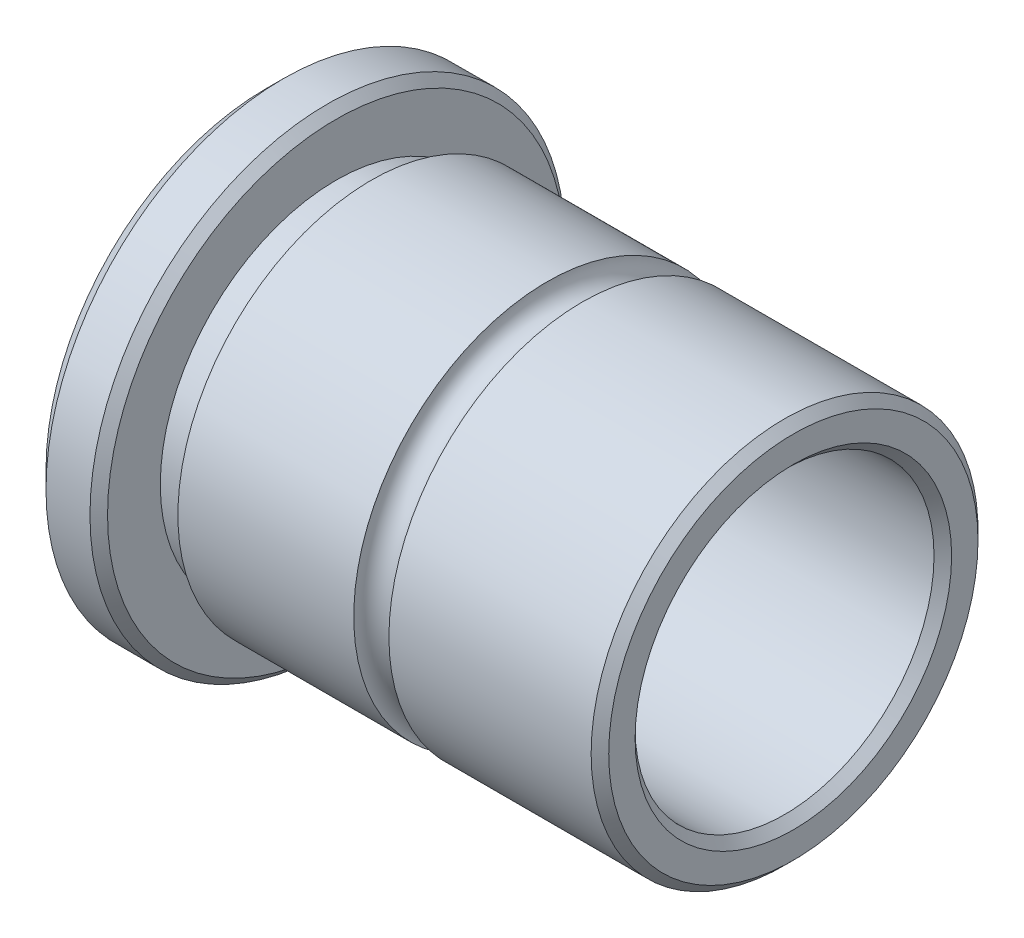
from build123d import *

# Parameters (mm, degrees)
CHAMFER1_SIZE = 1
CHAMFER2_SIZE = 0.5
SKETCH2_R     = 1


with BuildPart() as part:
    # Sketch1 → Revolve1 (revolve)
    with BuildSketch(Plane.XY, mode=Mode.PRIVATE) as revolve1_sk:
        Polygon((30, 8.5), (0, 8.5), (0, 13.5), (4, 13.5), (4, 11), (30, 11), align=None)
    revolve(revolve1_sk.sketch.rotate(Axis((0, 0, 0), (1, 0, 0)), 90), axis=Axis((0, 0, 0), (1, 0, 0)))

    # Chamfer1
    chamfer1_edges = [part.edges().sort_by_distance(p)[0] for p in [
        (0, 0, -13.5),
    ]]
    chamfer(chamfer1_edges, length=CHAMFER1_SIZE)

    # Chamfer2
    chamfer2_edges = [part.edges().sort_by_distance(p)[0] for p in [
        (30, 0, -11),
        (4, 0, -13.5),
        (0, 0, -8.5),
        (30, 0, -8.5),
    ]]
    chamfer(chamfer2_edges, length=CHAMFER2_SIZE)

    # Sketch2 → Cut-Revolve1 (revolve, cut)
    with BuildSketch(Plane(origin=(0, 0, 0), x_dir=(1, 0, 0), z_dir=(0, 1, 0))):
        with Locations((32, 11)):
            Circle(SKETCH2_R)
        with Locations((17, 11)):
            Circle(SKETCH2_R)
        Polygon((4, 11), (4, 10), (5.8, 10), (6, 11), align=None)
    revolve(axis=Axis((29.5, 0, 0), (-1, 0, 0)), mode=Mode.SUBTRACT)


solid = part.part
